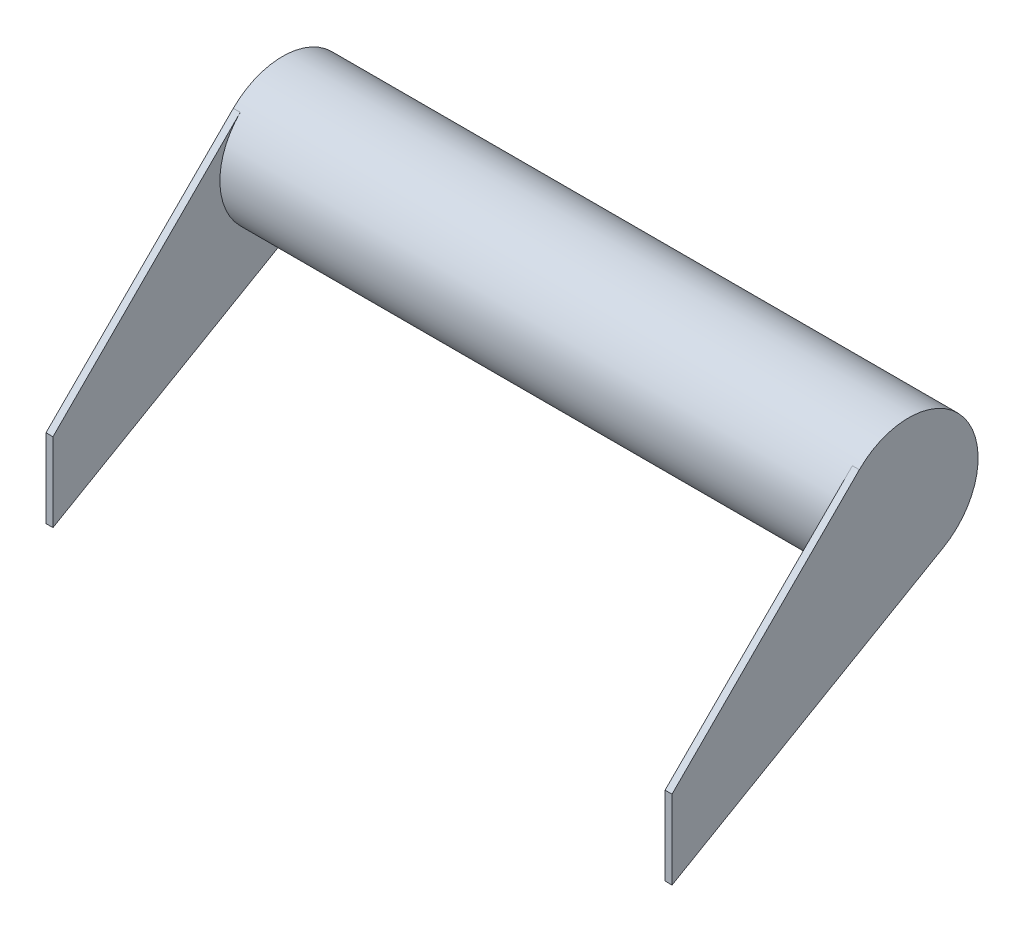
from build123d import *

# Parameters (mm, degrees)
SKETCH1_R           = 10
SKETCH1_R_2         = 9
BOSS_EXTRUDE1_DEPTH = 45
SKETCH2_R           = 10
SKETCH2_R_2         = 9
BOSS_EXTRUDE2_DEPTH = 1


with BuildPart() as part:
    # Sketch1 → Boss-Extrude1 (new, symmetric)
    with BuildSketch(Plane(origin=(0, 0, 0), x_dir=(0, 0, -1), z_dir=(1, 0, 0))):
        with Locations(Location((0, 0, 0), (0, 0, 180))):
            Circle(SKETCH1_R)
        with Locations(Location((0, 0, 0), (0, 0, 180))):
            Circle(SKETCH1_R_2, mode=Mode.SUBTRACT)
    extrude(amount=BOSS_EXTRUDE1_DEPTH, both=True)

    # Sketch2 → Boss-Extrude2 (add)
    # profile 1 of 3: a face of its own
    with BuildSketch(Plane(origin=(45, 0, 0), x_dir=(0, 0, -1), z_dir=(1, 0, 0))):
        with BuildLine():
            ThreePointArc((5, -8.660254038), (-7.933533403, -6.08761429), (-7.071067812, 7.071067812))
            Line((-7.071067812, 7.071067812), (-34, -19.857864376))
            Line((-34, -19.857864376), (-34, -31.176914536))
            Line((-34, -31.176914536), (5, -8.660254038))
        make_face()
    # profile 2 of 3: a face of its own
    with BuildSketch(Plane(origin=(45, 0, 0), x_dir=(0, 0, -1), z_dir=(1, 0, 0))):
        with Locations(Location((0, 0, 0), (0, 0, 135))):
            Circle(SKETCH2_R)
        with Locations(Location((0, 0, 0), (0, 0, 180))):
            Circle(SKETCH2_R_2, mode=Mode.SUBTRACT)
    # profile 3 of 3: a face of its own
    with BuildSketch(Plane(origin=(45, 0, 0), x_dir=(0, 0, -1), z_dir=(1, 0, 0))):
        with Locations(Location((0, 0, 0), (0, 0, 180))):
            Circle(SKETCH2_R_2)
    boss_extrude2 = extrude(amount=-BOSS_EXTRUDE2_DEPTH)

    # Mirror1: Boss-Extrude2 across plane
    add(boss_extrude2.mirror(Plane(origin=(0, 0, 0), x_dir=(0, 0, 1), z_dir=(1, 0, 0))))


solid = part.part
